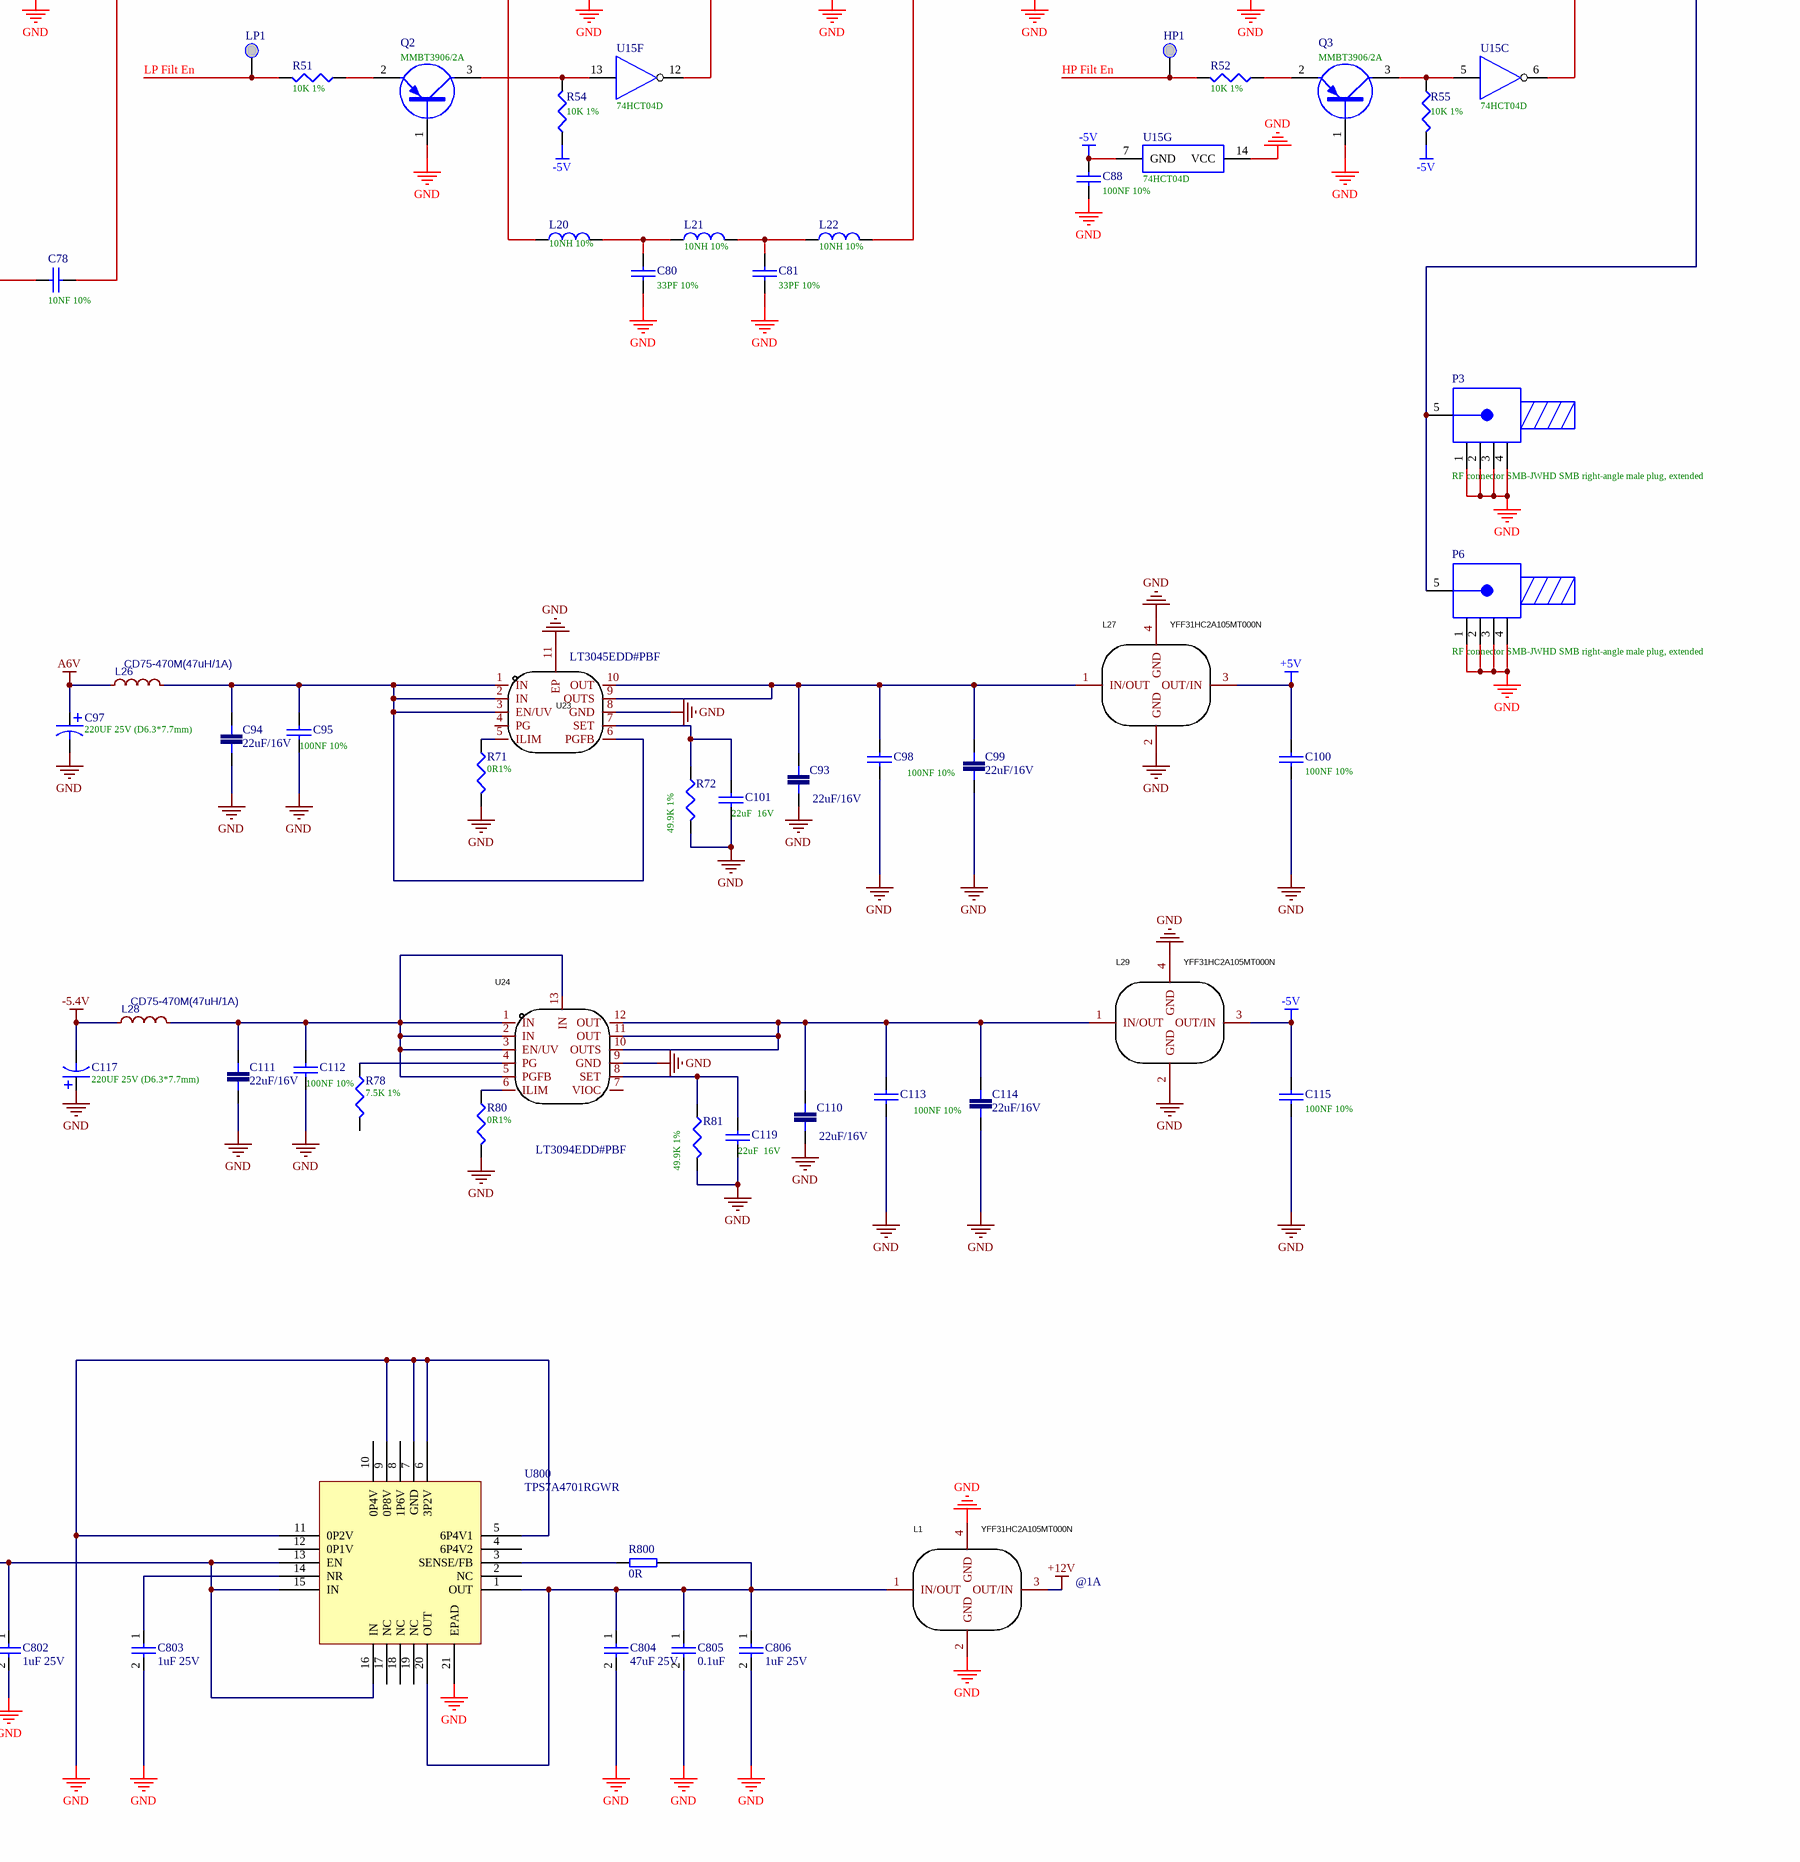
[diagram p0: PCBE109560-5.SchDoc, bottom right]
# Altium schematic sheet PCBE109560-5.SchDoc (part 2 of 2)

## Parts
1  (no value)  [DIP-1]
+1  (no value)  [DIP-1]
+2  (no value)  [DIP-1]
C4  20PF 10%  [0805C]
C5  330PF 10%  [1812C]
C6  22PF 10%  [1812C-2]
C7  22uF/16V  [0805]
C8  22uF/16V  [0805]
C9  100NF 10%  [0603]
C10  220UF 25V (D6.3*7.7mm)  [CAP-SMD_BD6.3-L6.6-W6.6-FD]
C11  100NF 10%  [0603]
C12  22uF/16V  [0805]
C13  100NF 10%  [0805R]
C14  22uF  16V  [0805]
C15  100NF 10%  [0805R]
C16  47PF 10%  [1812C-2]
C17  100PF 10%  [1812C-2]
C18  20PF 10%  [0805R]
C20  100NF 10%  [0805R]
C21  100NF 10%  [0805R]
C31  100NF 10%  [0805R]
C32  100NF 10%  [0805R]
C34  100NF 10%  [0805R]
C35  100NF 10%  [0805R]
C36  100NF 10%  [0805R]
C37  100NF 10%  [0805R]
C39  100NF 10%  [0805R]
C40  100NF 10%  [0805R]
C41  100NF 10%  [0805R]
C42  100NF 10%  [0805R]
C43  100NF 10%  [0805R]
C44  100NF 10%  [0805R]
C45  100NF 10%  [0805R]
C46  100NF 10%  [0805R]
C47  100NF 10%  [0805R]
C48  100NF 10%  [0805R]
C49  22uF 25V  [CAP-SMD_L6.0-W3.2-R-RD]
C50  100NF 10%  [0805R]
C51  100NF 10%  [0805R]
C52  100NF 10%  [0805R]
C53  3.3NF 10%  [0805R]
C54  100NF 10%  [0805R]
C55  330PF 10%  [0805R]
C56  330PF 10%  [0805R]
C57  100NF 10%  [0805R]
C58  33PF 10%  [0805R]
C59  33PF 10%  [0805R]
C60  100NF 10%  [0805R]
C61  100NF 10%  [0805R]
C62  100NF 10%  [0805R]
C63  100NF 10%  [0805R]
C64  100NF 10%  [0805R]
C65  33PF 10%  [0805R]
C66  33PF 10%  [0805R]
C67  100NF 10%  [0805R]
C68  39PF 10%  [0805R]
C69  100NF 10%  [0805R]
C70  25V 1UF Type A  [0805C-2]
C71  25V 1UF Type A  [0805C-2]
C72  100NF 10%  [0805R]
C73  25V 1UF Type A  [0805C-2]
C74  100NF 10%  [0805R]
C75  100NF 10%  [0805R]
C76  10NF 10%  [0805R]
C77  10NF 10%  [0805R]
C78  10NF 10%  [0805R]
C79  100NF 10%  [0603C]
C80  33PF 10%  [0805R]
C81  33PF 10%  [0805R]
C82  100NF 10%  [0805R]
C83  100NF 10%  [0805R]
C84  100NF 10%  [0805R]
C85  100NF 10%  [0805R]
C86  25V 1UF Type A  [0805C-2]
C87  3pF( ±0.1pF)  [0805R]
C88  100NF 10%  [0805R]
C89  100NF 10%  [0805R]
C90  100NF 10%  [0805R]
C93  22uF/16V  [0805]
C94  22uF/16V  [0805]
C95  100NF 10%  [0603]
C96  100NF 10%  [0805R]
C97  220UF 25V (D6.3*7.7mm)  [CAP-SMD_BD6.3-L6.6-W6.6-FD]
C98  100NF 10%  [0603]
C99  22uF/16V  [0805]
C100  100NF 10%  [0805R]
C101  22uF  16V  [0805]
C102  100NF 10%  [0805R]
C103  100NF 10%  [0805R]
C104  100NF 10%  [0805R]
C105  100NF 10%  [0805R]
C106  100NF 10%  [0805R]
C107  100NF 10%  [0805R]
C109  100NF 10%  [0805R]
C110  22uF/16V  [0805]
C111  22uF/16V  [0805]
C112  100NF 10%  [0603]
C113  100NF 10%  [0603]
C114  22uF/16V  [0805]
C115  100NF 10%  [0805R]
C116  100NF 10%  [0805R]
C117  220UF 25V (D6.3*7.7mm)  [CAP-SMD_BD6.3-L6.6-W6.6-FD]
C118  100NF 10%  [0805R]
C119  22uF  16V  [0805]
C122  100NF 10%  [0805R]
C123  100NF 10%  [0805R]
C124  100NF 10%  [0805R]
C125  100NF 10%  [0805R]
C128  100NF 10%  [0805R]
C129  100NF 10%  [0805R]
C130  100NF 10%  [0805R]
C800  47uF 25V  [1206]
C801  0.1uF  [0402]
C802  1uF 25V  [0402]
C803  1uF 25V  [0402]
C804  47uF 25V  [1206]
C805  0.1uF  [0402]
C806  1uF 25V  [0402]
Clk1  (no value)  [DIP-1]
D1  BAV99/A7  [SOT-23]
D2  GF1M-E3/67A/GM  [1808D]
D3  GF1M-E3/67A/GM  [1808D]
D4  GF1M-E3/67A/GM  [1808D]
D5  GF1M-E3/67A/GM  [1808D]
D8  BAV99/A7  [SOT-23-2]
D9  BAV99/A7  [SOT-23-2]
D10  BAV99/A7  [SOT-23-2]
D11  BAV99/A7  [SOT-23-2]
D12  BAV99/A7  [SOT-23-2]
Data1  (no value)  [DIP-1]
HP1  (no value)  [DIP-1]
J1  RF connector  [DIP-P]
J2  RF connector  [DIP-P]
L1  YFF31HC2A105MT000N  [FILTER-SMD_4P-L3.2-W1.6-L_YFF31HC]
L2  15UH 5%  [1005R]
L3  BLM21PG221SN1D(220Ω@100MHz)  [0805R]
L4  YFF31HC2A105MT000N  [FILTER-SMD_4P-L3.2-W1.6-L_YFF31HC]
L5  6.8UH 10%  [0805R]
L8  YFF31HC2A105MT000N  [FILTER-SMD_4P-L3.2-W1.6-L_YFF31HC]
L9  BLM21PG221SN1D(220Ω@100MHz  [0805R]
L10  10NH 10%  [0805R]
L11  10NH 10%  [0805R]
L12  10NH 10%  [0805R]
L13  YFF31HC2A105MT000N  [FILTER-SMD_4P-L3.2-W1.6-L_YFF31HC]
L14  BLM21PG221SN1D(220Ω@100MHz  [0805R]
L15  4.7UH 5%  [1005L]
L16  1UH 5%  [0805R]
L17  BLM21PG221SN1D(220Ω@100MHz)  [0805R]
L18  BLM21PG221SN1D(220Ω@100MHz  [0805R]
L19  BLM21PG221SN1D(220Ω@100MHz  [0805R]
L20  10NH 10%  [0805R]
L21  10NH 10%  [0805R]
L22  10NH 10%  [0805R]
L23  YFF31HC2A105MT000N  [FILTER-SMD_4P-L3.2-W1.6-L_YFF31HC]
L24  YFF31HC2A105MT000N  [FILTER-SMD_4P-L3.2-W1.6-L_YFF31HC]
L25  BLM21PG221SN1D(220Ω@100MHz  [0805R]
L26  CD75-470M(47uH/1A)  [IND-SMD_L7.8-W7.0-A]
L27  YFF31HC2A105MT000N  [FILTER-SMD_4P-L3.2-W1.6-L_YFF31HC]
L28  CD75-470M(47uH/1A)  [IND-SMD_L7.8-W7.0-A]
L29  YFF31HC2A105MT000N  [FILTER-SMD_4P-L3.2-W1.6-L_YFF31HC]
L31  BLM21PG221SN1D(220Ω@100MHz  [0805R]
L32  BLM21PG221SN1D(220Ω@100MHz  [0805R]
L808  NFM15PC104R1A3D  [FILTER-SMD_0402-3P-L1.0-W0.5-T]
L809  NFM15PC104R1A3D  [FILTER-SMD_0402-3P-L1.0-W0.5-T]
L810  NFM15PC104R1A3D  [FILTER-SMD_0402-3P-L1.0-W0.5-T]
L811  NFM15PC104R1A3D  [FILTER-SMD_0402-3P-L1.0-W0.5-T]
L812  NFM15PC104R1A3D  [FILTER-SMD_0402-3P-L1.0-W0.5-T]
L813  NFM15PC104R1A3D  [FILTER-SMD_0402-3P-L1.0-W0.5-T]
LP1  (no value)  [DIP-1]
P1  Header 20X2  [N0.8mm/40Pin-Plug]
P2  Header 4X2  [N0.8mm/8Pin-SOCKET]
P3  RF connector SMB-JWHD SMB right-angle male plug, extended  [DIP-P-2]
P4  Header 20X2  [N0.8mm/40Pin-Plug]
P5  Header 20X2  [N0.8mm/40Pin-Plug]
P6  RF connector SMB-JWHD SMB right-angle male plug, extended  [DIP-P-2]
Q1  MJD31C  [SOT-252-2]
Q2  MMBT3906/2A  [SOT-23]
Q3  MMBT3906/2A  [SOT-23]
Q4  MMBT3906/2A  [SOT-23]
R6  2K 5%  [0603R]
R7  NC  [AXIAL-0.51]
R8  3.9K 5% 1/2W  [AXIAL-0.51]
R9  3.9K 5% 1/2W  [AXIAL-0.51]
R10  3.9K 5% 1/2W  [AXIAL-0.51]
R11  3.9K 5% 1/2W  [AXIAL-0.51]
R13  0R1%  [0603]
R14  49.9K 1%  [0603]
R15  4.99K 1%  [0805R]
R16  2K 1%  [0805R]
R17  49.9R 1% 1/4W  [AXIAL-0.4]
R20  100R 1% 1/4W  [AXIAL-0.4]
R23  100R 1% 1/4W  [AXIAL-0.4]
R27  4.87K 1%  [0805R]
R28  4.87K 1%  [0805R]
R29  4.87K 1%  [0805R]
R30  4.87K 1%  [0805R]
R31  4.87K 1%  [0805R]
R32  10K 1%  [0805R]
R33  100K 1%  [0805R]
R34  100K 1%  [0805R]
R35  49.9R 1%  [0805R]
R36  49.9R 1%  [0805R]
R37  49.9R 1%  [0805R]
R38  49.9R 1%  [0805R]
R39  49.9R 1%  [0805R]
R40  49.9R 1% 1/4W  [R-SMD_L3.5-W1.5]
R41  10K 1%  [0805R]
R42  4.87K 1%  [0805R]
R43  4.87K 1%  [0805R]
R44  4.87K 1%  [0805R]
R45  4.87K 1%  [0805R]
R46  169R 1%  [0805R]
R47  169R 1%  [0805R]
R48  169R 1%  [0805R]
R49  49.9R 1%  [0805R]
R50  49.9R 1%  [0805R]
R51  10K 1%  [0805R]
R52  10K 1%  [0805R]
R53  10K 1%  [0805R]
R54  10K 1%  [0805R]
R55  10K 1%  [0805R]
R56  10K 1%  [0805R]
R57  10K 1%  [0805R]
R58  49.9R 1%  [0805R]
R59  4.99K 1%  [0805R]
R60  49.9R 1%  [R-SMD_L3.5-W1.5]
R61  30R 1%  [R-SMD_L3.5-W1.5]
R62  169R 1%  [0805R]
R63  169R 1%  [0805R]
R64  169R 1%  [0805R]
R65  49.9R 1%  [0805R]
R66  49.9R 1%  [0805R]
R67  49.9R 1%  [0805R]
R68  49.9R 1%  [0805R]
R69  120R 1%  [R-SMD_L3.5-W1.5]
R70  169R 1%  [0805R]
R71  0R1%  [0603]
R72  49.9K 1%  [0603]
R73  169R 1%  [0805R]
R74  NC  [0805R]
R75  169R 1%  [0805R]
R77  169R 1%  [0805R]
R78  7.5K 1%  [0603]
R80  0R1%  [0603]
R81  49.9K 1%  [0603]
R82  100K 1%  [0805R]
R83  10K 1%  [0805R]
R84  169R 1%  [0805R]
R800  0R  [0402]
RE1  AGQ210A4HZ  [RELAY-SMD_PANASONIC_AGQ2X0AXX]
RE2  AGQ210A4HZ  [RELAY-SMD_PANASONIC_AGQ2X0AXX]
RE3  AGQ210A4HZ  [RELAY-SMD_PANASONIC_AGQ2X0AXX]
RE4  AGQ210A4HZ  [RELAY-SMD_PANASONIC_AGQ2X0AXX]
RE5  AGQ210A4HZ  [RELAY-SMD_PANASONIC_AGQ2X0AXX]
Strobe1  (no value)  [DIP-1]
U4  LT3045EDD#PBF  [DFN-10_L3.0-W3.0-P0.50-BL-EP]
U6  74HCT123D  [SOIC-16_L9.9-W3.9-P1.27-LS6.0-BL]
U8  MAX504CSD+T  [SO-14]
U9  SW-239  [SO-8]
U11  SW-239  [SO-8]
U12  SW-239  [SO-8]
U13  SW-239  [SO-8]
U14  SW-239  [SO-8]
U15  74HCT04D  [SO-14]  (parts A,B,C,D,E,F,G of 7)
U16  AT-250(MAAV-007941)  [SO-8]
U17  MAR-3SM/A03  [LCC4]
U18  MAR-6SM/A06  [LCC4]
U19  MAR-6SM/A06  [LCC4]
U20  MAR-3SM/A03  [LCC4]
U21  MAX4106ESA+T  [SO-8]
U22  MIC4420CM  [SO-8]
U23  LT3045EDD#PBF  [DFN-10_L3.0-W3.0-P0.50-BL-EP]
U24  LT3094EDD#PBF  [WDFN-12_L3.0-W3.0-P0.45-BL-EP]
U25  AT65-0263  [SO-16]
U100  SW-239  [SO-8]
U800  TPS7A4701RGWR  [QFN-20]

## Nets
+5V: C100.1 L27.3(OUT/IN) L808.3(OUTPUT) L811.3(OUTPUT) L812.3(OUTPUT) U8.3(~{CLR})
+12.5V: +2.1 C106.1 C800.1 C801.1 C802.1 P5.31 P5.32 P5.33 P5.34 P5.35 P5.36 P5.37 P5.38 P5.39 P5.40 U800.13(EN) U800.15(IN) U800.16(IN)
+12V: C122.1 C123.1 C124.2 C125.2 L1.3(OUT/IN) L8.1(IN/OUT) L13.1(IN/OUT) U22.1(VS) U22.8(VS)
-5.4V: +1.1 C107.1 C117.2 L28.2 P5.1 P5.2 P5.3 P5.4 P5.5 P5.6 P5.7 P5.8 P5.9 P5.10
-5V: C88.2 C115.2 L29.3(OUT/IN) L809.1(INPUT) L810.3(OUTPUT) L813.3(OUTPUT) R54.1 R55.2 R57.1 U15.7(GND)
A6V: 1.1 C10.1 C97.1 C103.2 L3.1 L26.2 P5.17 P5.18 P5.19 P5.20 P5.21 P5.22 P5.23 P5.24
GND: C5.1 C6.2 C7.1 C8.1 C9.2 C10.2 C11.2 C12.1 C13.2 C14.2 C15.1 C18.2 C20.1 C21.1 C31.1 C32.1 C34.1 C35.1 C36.2 C37.2 C39.2 C40.2 C42.2 C43.1 C44.2 C45.2 C46.2 C47.1 C48.1 C49.2 C50.2 C57.2 C60.2 C61.1 C62.1 C63.1 C64.1 C65.2 C66.1 C70.1 C71.1 C72.2 C73.1 C74.1 C75.1 C80.1 C81.1 C83.2 C84.2 C85.1 C86.2 C88.1 C89.2 C90.2 C93.1 C94.1 C95.2 C96.2 C97.2 C98.2 C99.1 C100.2 C101.2 C102.2 C103.1 C104.2 C105.1 C106.2 C107.2 C109.2 C110.1 C111.1 C112.2 C113.2 C114.1 C115.1 C117.1 C118.2 C119.2 C122.2 C123.2 C124.1 C125.1 C128.1 C129.1 C130.2 C800.2 C801.2 C802.2 C803.2 C804.2 C805.2 C806.2 D1.3 D2.2(K) D11.2 D12.1 J1.1 J1.2 J1.3 J1.4 J2.1 J2.2 J2.3 J2.4 L1.2(GND) L1.4(GND) L2.2 L4.2(GND) L4.4(GND) L8.2(GND) L8.4(GND) L13.2(GND) L13.4(GND) L15.2 L16.1 L23.2(GND) L23.4(GND) L24.2(GND) L24.4(GND) L27.2(GND) L27.4(GND) L29.2(GND) L29.4(GND) L808.2(GND) L809.2(GND) L810.2(GND) L811.2(GND) L812.2(GND) L813.2(GND) P1.5 P1.6 P1.11 P1.12 P1.17 P1.18 P1.20 P1.23 P1.24 P1.29 P1.30 P1.35 P1.36 P2.1 P2.3 P2.5 P2.7 P3.1 P3.2 P3.3 P3.4 P4.5 P4.6 P4.11 P4.12 P4.17 P4.18 P4.23 P4.24 P4.29 P4.30 P4.35 P4.36 P5.11 P5.12 P5.13 P5.14 P5.15 P5.16 P5.25 P5.26 P5.27 P5.28 P5.29 P5.30 P6.1 P6.2 P6.3 P6.4 Q1.2(E) Q2.1(B) Q3.1(B) Q4.1(B) R13.2 R14.2 R20.2 R32.2 R53.1 R59.1 R61.1 R71.2 R72.2 R74.1 R80.2 R81.2 R82.1 R83.1 RE1.3 RE3.6 RE4.2 U4.8(GND) U4.11(EP) U6.6(2CEXT) U6.8(GND) U6.10(2B) U6.14(1CEXT) U8.7(DGND) U8.8(AGND) U9.2(GND) U9.7(GND) U9.8(GND) U11.2(GND) U11.7(GND) U11.8(GND) U12.2(GND) U12.7(GND) U12.8(GND) U13.2(GND) U13.7(GND) U13.8(GND) U14.2(GND) U14.7(GND) U14.8(GND) U15.14(VCC) U16.2(GND) U16.3(GND) U16.5(GND) U16.6(GND) U16.7(GND) U17.2(GND) U17.4(GND) U18.2(GND) U18.4(GND) U19.2(GND) U19.4(GND) U20.2(GND) U20.4(GND) U22.4(GND) U22.5(GND) U23.8(GND) U23.11(EP) U24.9(GND) U25.2(GND) U25.3(GND) U25.4(GND) U25.5(GND) U25.6(GND) U25.7(GND) U25.16(GND) U100.2(GND) U100.7(GND) U100.8(GND) U800.5(6P4V1) U800.6(3P2V) U800.7(GND) U800.9(0P8V) U800.11(0P2V) U800.21(EPAD)
VCC: C13.1 C15.2 L4.3(OUT/IN) R15.1 R16.2 U6.2(1B) U6.3(1~{R}D) U6.16(VCC)
AK2: C21.2 P1.33 RE1.1
AK3: C20.2 P1.38 RE1.8
AK4: C37.1 P1.37 RE2.1
AK5: C36.1 P1.40 RE2.8
AK6: C31.2 P1.34 RE3.8
AK7: C32.2 P1.32 RE3.1
AK8: C34.2 C40.1 P1.28 RE4.8 RE5.8
AK9: C35.2 C39.1 P1.26 RE4.1 RE5.1
Attn1: P4.34 R70.2
Attn2: P4.32 R73.2
Attn4: P4.28 R75.2
Attn8: P4.26 R77.2
Attn16: P4.22 R84.2
DAC Clk: Clk1.1 P4.14 U8.4(SCLK)
DAC Data: Data1.1 P4.16 U8.2(DIN)
DAC Strobe: P4.10 Strobe1.1 U8.5(~{CS})
DATA_T: P1.39 R15.2 U6.1(1~{A})
HP Filt En: HP1.1 P4.4 R52.2
HT: L5.1 P2.2 P2.4 P2.6 P2.8
IN2: P4.8 R56.1 U22.2(IN)
LP Filt En: LP1.1 P4.2 R51.2
NetC4_1: C4.1 D1.2 L2.1 Q1.1(B) R6.1
NetC4_2: C4.2 R6.2 U6.13(1Q)
NetC5_2: C5.2 L5.2 R7.2
NetC6_1: C6.1 C16.2 C17.2 Q1.3(C) R11.1
NetC7_2: C7.2 C11.1 C12.2 L4.1(IN/OUT) U4.9(OUTS) U4.10(OUT)
NetC8_2: C8.2 C9.1 L3.2 U4.1(IN) U4.2(IN) U4.3(EN/UV) U4.6(PGFB)
NetC14_1: C14.1 R14.1 U4.7(SET)
NetC16_1: C16.1 D5.1(A) D8.2 D9.2 RE2.6
NetC17_1: C17.1 RE2.7
NetC18_1: C18.1 R16.1 U6.15(1REXT/CEXT)
NetC41_1: C41.1 U14.1(RFCOM)
NetC41_2: C41.2 P3.5 P6.5 R32.1
NetC42_1: C42.1 R27.1 U9.5(B)
NetC43_2: C43.2 R28.2 U100.4(A)
NetC44_1: C44.1 R29.1 U11.4(A)
NetC45_1: C45.1 R30.1 U12.5(B)
NetC46_1: C46.1 R31.1 U13.5(B) U14.4(A)
NetC47_2: C47.2 R35.1 U16.4(A)
NetC48_2: C48.2 L8.3(OUT/IN) R36.1
NetC49_1: C49.1 C50.1 U8.1(BIPOFF) U8.9(REFIN) U8.10(REFOUT)
NetC51_1: C51.1 U17.1(RF_IN)
NetC51_2: C51.2 U16.8(RF2)
NetC52_1: C52.1 L10.2
NetC52_2: C52.2 L9.1 U17.3(RF_OUT)
NetC53_1: C53.1 C54.1 L15.1
NetC53_2: C53.2 U12.1(RFCOM)
NetC54_2: C54.2 U13.1(RFCOM)
NetC55_1: C55.1 U13.3(RF1)
NetC55_2: C55.2 C56.1 L16.2
NetC56_2: C56.2 U14.6(RF2)
NetC57_1: C57.1 R41.1 U13.4(A) U14.5(B)
NetC58_1: C58.1 C65.1
NetC58_2: C58.2 L10.1 L11.1
NetC59_1: C59.1 L11.2 L12.1
NetC59_2: C59.2 C66.2
NetC60_1: C60.1 R42.1 U9.4(A)
NetC61_2: C61.2 R43.2 U100.5(B)
NetC62_2: C62.2 R44.1 U11.5(B)
NetC63_2: C63.2 R45.1 U12.4(A)
NetC64_2: C64.2 L13.3(OUT/IN) R46.2
NetC67_1: C67.1 U18.1(RF_IN)
NetC67_2: C67.2 U25.1(RF)
NetC68_1: C68.1 C69.2 R49.2 R50.2
NetC68_2: C68.2 L14.2 R49.1 R50.1 U18.3(RF_OUT)
NetC69_1: C69.1 R53.2 U16.1(RF1)
NetC70_2: C70.2 C74.2 L18.1 L19.2
NetC71_2: C71.2 C75.2 L19.1 U21.4(VEE)
NetC72_1: C72.1 C73.2 L17.2 L18.2
NetC76_1: C76.1 U9.3(RF1)
NetC76_2: C76.2 U19.1(RF_IN)
NetC77_1: C77.1 R64.1 U19.3(RF_OUT)
NetC77_2: C77.2 U20.1(RF_IN)
NetC78_1: C78.1 R68.2 U20.3(RF_OUT)
NetC78_2: C78.2 U100.6(RF2)
NetC79_1: C79.1 D10.3 R40.2
NetC79_2: C79.2 R58.2 R59.2
NetC80_2: C80.2 L20.2 L21.2
NetC81_2: C81.2 L21.1 L22.1
NetC82_1: C82.1 R60.2
NetC82_2: C82.2 C116.1 R74.2 R82.2
NetC83_1: C83.1 C86.1 L25.2 U21.7(VCC)
NetC84_1: C84.1 L23.3(OUT/IN) R62.2
NetC85_2: C85.2 L24.3(OUT/IN) R65.1
NetC87_1: C87.1 R60.1 R69.1 U21.6(OUT)
NetC87_2: C87.2 R61.2 R69.2 U21.2(IN-)
NetC89_1: C89.1 L813.1(INPUT) U8.11(VSS)
NetC90_1: C90.1 L32.2 L811.1(INPUT)
NetC93_2: C93.2 C98.1 C99.2 L27.1(IN/OUT) U23.9(OUTS) U23.10(OUT)
NetC94_2: C94.2 C95.1 L26.1 U23.1(IN) U23.2(IN) U23.3(EN/UV) U23.6(PGFB)
NetC96_1: C96.1 R70.1 U25.15(C1)
NetC101_1: C101.1 R72.1 U23.7(SET)
NetC102_1: C102.1 R73.1 U25.14(C2)
NetC104_1: C104.1 L812.1(INPUT) U8.13(VDD)
NetC105_2: C105.2 L31.1 L810.1(INPUT)
NetC109_1: C109.1 R75.1 U25.13(C4)
NetC110_2: C110.2 C113.1 C114.2 L29.1(IN/OUT) U24.10(OUTS) U24.11(OUT) U24.12(OUT)
NetC111_2: C111.2 C112.1 L28.1 U24.1(IN) U24.2(IN) U24.3(EN/UV) U24.5(PGFB) U24.13(IN)
NetC116_2: C116.2 R83.2 U25.8(RF)
NetC118_1: C118.1 R77.1 U25.12(C8)
NetC119_1: C119.1 R81.1 U24.8(SET)
NetC128_2: C128.2 L31.2 U25.11(VEE)
NetC129_2: C129.2 L32.1 U25.10(VCC)
NetC130_1: C130.1 R84.1 U25.9(C16)
NetC803_1: C803.1 U800.14(NR)
NetC804_1: C804.1 C805.1 C806.1 L1.1(IN/OUT) R800.1 U800.1(OUT) U800.20(OUT)
NetD2_1: D2.1(A) D3.2(K)
NetD3_1: D3.1(A) D4.2(K)
NetD4_1: D4.1(A) D5.2(K)
NetD8_1: D8.1 D9.1 J1.5 R17.1 R20.1 R23.1 RE4.4
NetD10_1: D10.1 D12.2
NetD10_2: D10.2 D11.1
NetJ2_5: J2.5 RE5.4
NetL9_2: L9.2 R39.2
NetL12_2: L12.2 U9.1(RFCOM)
NetL14_1: L14.1 R48.2
NetL17_1: L17.1 L809.3(OUTPUT)
NetL20_1: L20.1 U11.6(RF2)
NetL22_2: L22.2 U12.3(RF1)
NetL23_1: L23.1(IN/OUT) L24.1(IN/OUT) U22.6(OUT) U22.7(OUT)
NetL25_1: L25.1 L808.1(INPUT)
NetQ2_2: Q2.2(E) R51.1
NetQ2_3: Q2.3(C) R54.2 U15.13(6A)
NetQ3_2: Q3.2(E) R52.1
NetQ3_3: Q3.3(C) R55.1 U15.5(3A)
NetQ4_2: Q4.2(E) R56.2
NetQ4_3: Q4.3(C) R57.2 U15.1(1A)
NetR7_1: R7.1 R8.1
NetR8_2: R8.2 R9.2
NetR9_1: R9.1 R10.1
NetR10_2: R10.2 R11.2
NetR13_1: R13.1 U4.5(ILIM)
NetR17_2: R17.2 RE1.2
NetR23_2: R23.2 RE3.7
NetR27_2: R27.2 R28.1 U15.4(2Y)
NetR29_2: R29.2 R30.2 U15.10(5Y)
NetR31_2: R31.2 U15.8(4Y)
NetR33_1: R33.1 R34.1 U8.14(RFB)
NetR33_2: R33.2 R34.2 R35.2 U8.12(VOUT)
NetR36_2: R36.2 R37.1
NetR37_2: R37.2 R38.2
NetR38_1: R38.1 R39.1
NetR40_1: R40.1 RE5.3
NetR41_2: R41.2 U15.6(3Y) U15.9(4A)
NetR42_2: R42.2 R43.1 U15.2(1Y) U15.3(2A)
NetR44_2: R44.2 R45.2 U15.11(5A) U15.12(6Y)
NetR46_1: R46.1 R47.2
NetR47_1: R47.1 R48.1
NetR58_1: R58.1 U21.3(IN+)
NetR62_1: R62.1 R63.1
NetR63_2: R63.2 R64.2
NetR65_2: R65.2 R66.2
NetR66_1: R66.1 R67.1
NetR67_2: R67.2 R68.1
NetR71_1: R71.1 U23.5(ILIM)
NetR78_1: R78.1 U24.4(PG)
NetR80_1: R80.1 U24.6(ILIM)
NetR800_2: R800.2 U800.3(SENSE/FB)
NetRE4_3: RE4.3 RE5.2
NetU9_6: U9.6(RF2) U100.3(RF1)
NetU11_1: U11.1(RFCOM) U100.1(RFCOM)
NetU11_3: U11.3(RF1) U12.6(RF2)
NetU13_6: U13.6(RF2) U14.3(RF1)

Not connected (* = marked no-connect by the designer): D1 1*; D8 3; D9 3; D11 3; D12 3; P1 1 2 3 4 7 8 9 10 13 14 15 16 19 21 22 25 27 31; P4 1 3 7 9 13 15 19 20 21 25 27 31 33 37 38 39 40; R78 2; RE1 4 5 6 7; RE2 2 3 4 5; RE3 2 3 4 5; RE4 5 6 7; RE5 5 6 7; U4 4(PG); U6 4(1~{Q}) 5(2Q) 7(2REXT/CEXT) 9(2~{A}) 11(2~{R}D) 12(2~{Q}); U8 6(DOUT); U22 3(NC); U23 4(PG); U24 7(VIOC); U800 2(NC) 4(6P4V2) 8(1P6V) 10(0P4V) 12(0P1V) 17(NC) 18(NC) 19(NC)

## Notes on the sheet
- (near P1) Transmit interface
- 500V high-voltage interface
- Receive interface
- @1A

## Library data of the parts
1 +1 +2 Clk1 Data1 HP1 LP1 Strobe1 = TP
C4-C6 C9 C11 C13-C18 C20 C21 C31 C32 C34-C37 C39-C48 C50-C69 C72-C85 C87-C90 C95 C96 C98 C100-C107 C109 C112 C113 C115 C116 C118 C119 C122-C125 C128-C130 C800-C806 = CAP: Capacitor
C7 C8 C12 C93 C94 C99 C110 C111 C114 = C1206
C10 C97 C117 = CAPACITOR_1: Capacitor
C49 = TAJC226K025RNJ: Manufacturer: Kyocera AVX; Add into BOM: yes; Tolerance: ±10%; Equivalent Series Resistance(ESR): 1.4Ω@100kHz; Symbol: TAJC226K025RNJ; Device: TAJC226K025RNJ; LCSC Part Name: 22uF ±10% 25V; Supplier Part: C7214; Manufacturer Part: TAJC226K025RNJ; Supplier Footprint: CASE-C-6032; JLCPCB Part Class: Extended Part; Datasheet: https://atta.szlcsc.com/upload/public/pdf/source/20160107/1457707750344.pdf; Supplier: LCSC; Convert to PCB: yes; Value: 22uF; Rated Voltage: 25V; Operating Temperature: -55℃~+125℃
C70 C71 C86 = CAPACITOR POL: Capacitor
D1 D8-D12 = BAV99
D2-D5 = DIODE
J1 J2 = SMA-KWE: BOM_Supplier: *; BOM_Supplier Part: *; BOM_Manufacturer: *; BOM_Manufacturer Part: *; BOM_JLCPCB Part Class: *; spicePre: *; spiceSymbolName: *; Contributor: *
L1 L4 L8 L13 L23 L24 L27 L29 = YFF31HC2A105MT000N: Manufacturer: TDK; Add into BOM: yes; Nominal Capacitance: 1uF; CapacitanceTolerance: ±20%; DC Rated Voltage: 100V; Rated Current: 6A; DC Resistance: 5mΩ; Name: YFF31HC2A105MT000N; Symbol: YFF31HC2A105MT000N; Device: YFF31HC2A105MT000N; LCSC Part Name: 1uF(105) ±20% 100V; Supplier Part: C113216; Manufacturer Part: YFF31HC2A105MT000N; Supplier Footprint: SMD-4P,1.6x3.2mm; JLCPCB Part Class: Extended Part; Datasheet: https://atta.szlcsc.com/upload/public/pdf/source/20180326/C113216_F6F81E50B9805DA3D7C436129903DEBD.pdf; Supplier: LCSC; Convert to PCB: yes; Operating Temperature: -55℃~+125℃
L2 L3 L5 L9-L12 L14-L22 L25 L31 L32 = INDUCTOR
L26 L28 = 4.7uH/5a: BOM_Manufacturer: COILMX; BOM_Manufacturer Part: MS0630-4R7M; nameAlias: Inductance; Contributor: LCSC; BOM_Supplier: LCSC; BOM_Supplier Part: C380177; spicePre: L; spiceSymbolName: MS0630-4R7M
L808-L813 = NFM15PC104R1A3D: Manufacturer: muRata(村田); Add into BOM: yes; Nominal Capacitance: 100nF; CapacitanceTolerance: ±20%; DC Rated Voltage: 10V; Rated Current: 2A; DC Resistance: 30mΩ; Symbol: NFM15PC104R1A3D; Device: NFM15PC104R1A3D; LCSC Part Name: 0.1uF ±20% 10V; Supplier Part: C2650905; Manufacturer Part: NFM15PC104R1A3D; Supplier Footprint: 0402; JLCPCB Part Class: Extended Part; Datasheet: https://atta.szlcsc.com/upload/public/pdf/source/20210611/05FD8D968916F804F398094FB2B4AAFE.pdf; Supplier: LCSC; Convert to PCB: yes; Operating Temperature: -55℃~+105℃; Comment_1: NFM15PC104R1A3D
P1 P4 P5 = Header 20X2: Header, 20-Pin, Dual row; LatestRevisionDate: 17-Jul-2002; LatestRevisionNote: Re-released for DXP Platform.; Publisher: Altium Limited
P2 = Header 4X2: Header, 4-Pin, Dual row; LatestRevisionDate: 17-Jul-2002; LatestRevisionNote: Re-released for DXP Platform.; Publisher: Altium Limited
P3 P6 = JA1
Q1 = NPN: NPN Transistor
Q2-Q4 = PNP: PNP Transistor
R6-R11 R13-R17 R20 R23 R27-R75 R77 R78 R80-R84 = RES1
R800 = RES
RE1-RE5 = AGQ210A4HZ: Manufacturer: PANASONIC(松下); Add into BOM: yes; Coil Voltage: 4.5V; Contact Form: Two changeover sets: 2C (DPDT changeover); Maximum Switching Voltage: 125V@AC; 110V@DC; Coil Type: Single coil; Maximum Switching Current: 2A; Operate Time: 4ms; Symbol: AGQ210A4HZ; Device: AGQ210A4HZ; LCSC Part Name: AGQ210A4HZ; Supplier Part: C2153577; Manufacturer Part: AGQ210A4HZ; Supplier Footprint: SMD,7.2x10.6mm; JLCPCB Part Class: Extended Part; Datasheet: https://atta.szlcsc.com/upload/public/pdf/source/20210727/C2858037_82AE1FE69E1888D41D6E9B5D42950540.pdf; Supplier: LCSC; Convert to PCB: yes; Pin Number: -; Contact Rating: -; Contact Material: AgPd + gold plating; Coil Rated Power: -; Coil Resistance: -; Release Time: 4ms; Contact Resistance: -; Operating Temperature: -40℃~+85℃; Comment_1: AGQ210A4HZ
U4 U23 = LT3045EDD#PBF: Symbol: LT3045EDD#PBF_C666574; Add into BOM: yes; Maximum Input Voltage: 20V; Output Voltage: 0V~15V; MAX Output Current: 500mA; Dropout Voltage: 450mV@(500mA); standby current: 20uA; Number of Outputs: 1; Device: LT3045EDD#PBF; LCSC Part Name: LT3045EDD#PBF; Supplier Part: C666574; Manufacturer Part: LT3045EDD#PBF; Supplier Footprint: DFN-10-EP(3x3); JLCPCB Part Class: Extended Part; Datasheet: https://atta.szlcsc.com/upload/public/pdf/source/20200416/C514420_E440C492D6C74EAE6AB301243586F696.pdf; Supplier: LCSC; Convert to PCB: yes
U15 = 74HC04
U16 = AT-250
U17 U20 = MAR-3SM
U18 U19 = MAR-6SM
U21 = MAX4107ESA: Manufacturer: *; Manufacturer Part: *; Supplier Part: *; Supplier: *; link: *; spicePre: *; spiceSymbolName: *; Package Display: *; Contributor: *
U24 = LT3094EDD#PBF: Add into BOM: yes; Symbol: LT3094EDD#PBF; Device: LT3094EDD#PBF; LCSC Part Name: LT3094EDD#PBF; Supplier Part: C670492; Manufacturer Part: LT3094EDD#PBF; Supplier Footprint: WDFN-12-EP(3x3); JLCPCB Part Class: Extended Part; Datasheet: https://atta.szlcsc.com/upload/public/pdf/source/20200318/C498217_A5485280C797CF3891C55BEBE66C21D4.pdf; Supplier: LCSC; Convert to PCB: yes; Output Type: -
U800 = TPS7A4701RGWR(QFN20): Name: *; Symbol: *; Device: *; LCSC Part Name: *; Supplier Part: *; Manufacturer: *; Manufacturer Part: *; Supplier Footprint: *; JLCPCB Part Class: *; Datasheet: *; Supplier: *; Add into BOM: *; Convert to PCB: *; Output Type: *; Output Polarity: *; Number of Outputs: *